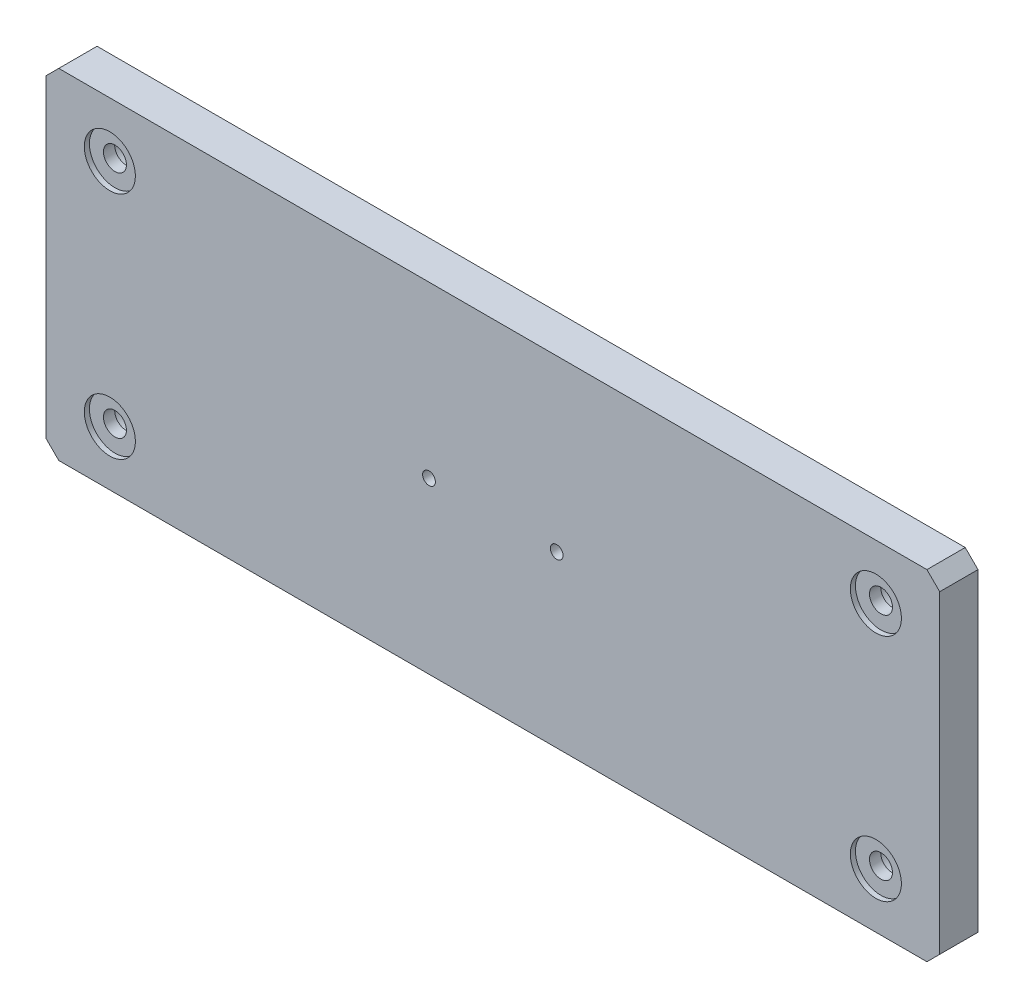
from build123d import *

# Parameters (mm, degrees)
SKETCH1_W                                           = 350
SKETCH1_H                                           = 133
BOSS_EXTRUDE1_DEPTH                                 = 7.5
CBORE_FOR_M8_HEX_SOCKET_HEAD_CAP_SCREW1_D           = 9
CBORE_FOR_M8_HEX_SOCKET_HEAD_CAP_SCREW1_CBORE_D     = 15
CBORE_FOR_M8_HEX_SOCKET_HEAD_CAP_SCREW1_CBORE_DEPTH = 8.6
M6_TAPPED_HOLE1_D                                   = 5
SKETCH6_R                                           = 10
CUT_EXTRUDE1_DEPTH                                  = 2
M4_TAPPED_HOLE1_D                                   = 3.3
M4_TAPPED_HOLE1_DEPTH                               = 10.1
M4_TAPPED_HOLE1_TIP                                 = 0.991420021
CHAMFER1_SIZE                                       = 5


with BuildPart() as part:
    # Sketch1 → Boss-Extrude1 (new, symmetric)
    with BuildSketch(Plane.XY):
        Rectangle(SKETCH1_W, SKETCH1_H)
    extrude(amount=BOSS_EXTRUDE1_DEPTH, both=True)

    # CBORE for M8 Hex Socket Head Cap Screw1 (through all)
    with Locations(Plane(origin=(0, 0, -7.5), x_dir=(-1, 0, 0), z_dir=(0, 0, -1))):
        with Locations((-150, 45), (-150, -45), (150, -45), (150, 45)):
            CounterBoreHole(CBORE_FOR_M8_HEX_SOCKET_HEAD_CAP_SCREW1_D / 2, CBORE_FOR_M8_HEX_SOCKET_HEAD_CAP_SCREW1_CBORE_D / 2, CBORE_FOR_M8_HEX_SOCKET_HEAD_CAP_SCREW1_CBORE_DEPTH)

    # M6 Tapped Hole1 (through all)
    with Locations(Plane.XY.offset(7.5)):
        with Locations((-25, 0), (25, 0)):
            Hole(M6_TAPPED_HOLE1_D / 2)

    # Sketch6 → Cut-Extrude1 (cut)
    with BuildSketch(Plane.XY.offset(7.5)):
        with Locations((-150, 45)):
            Circle(SKETCH6_R)
        with Locations(Location((-150, -45, 0), (0, 0, 180))):
            Circle(SKETCH6_R)
        with Locations((150, -45)):
            Circle(SKETCH6_R)
        with Locations(Location((150, 45, 0), (0, 0, 180))):
            Circle(SKETCH6_R)
    extrude(amount=-CUT_EXTRUDE1_DEPTH, mode=Mode.SUBTRACT)

    # M4 Tapped Hole1
    with Locations(Plane.ZY.offset(175)):
        with Locations((0, 14), (0, -1)):
            Hole(M4_TAPPED_HOLE1_D / 2, depth=M4_TAPPED_HOLE1_DEPTH)
            with Locations((0, 0, -(M4_TAPPED_HOLE1_DEPTH + M4_TAPPED_HOLE1_TIP / 2))):  # 118° drill point
                Cone(0, M4_TAPPED_HOLE1_D / 2, M4_TAPPED_HOLE1_TIP, mode=Mode.SUBTRACT)

    # Chamfer1
    chamfer1_edges = [part.edges().sort_by_distance(p)[0] for p in [
        (175, -66.5, 0),
        (-175, -66.5, 0),
        (-175, 66.5, 0),
        (175, 66.5, 0),
    ]]
    chamfer(chamfer1_edges, length=CHAMFER1_SIZE)


solid = part.part
